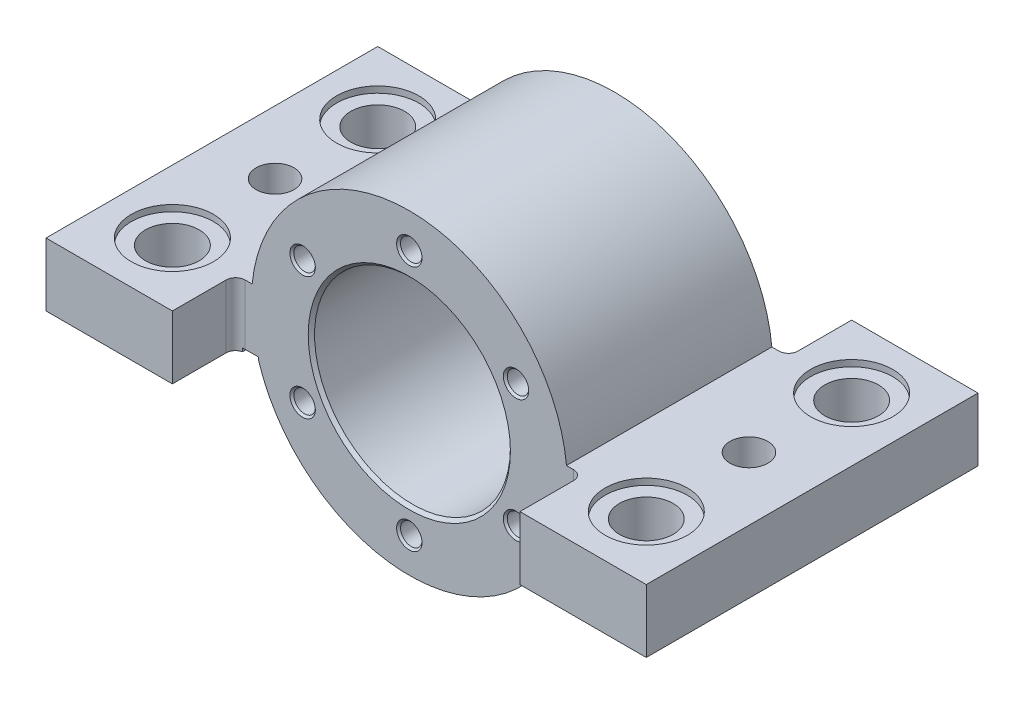
from build123d import *

# Parameters (mm, degrees)
BOSS_EXTRUDE1_DEPTH         = 52.5
BOSS_EXTRUDE1_DEPTH_BACK    = 52.5
SKETCH3_W                   = 5
SKETCH3_H                   = 10
CUT_EXTRUDE1_DEPTH          = 105
CUT_EXTRUDE2_DEPTH          = 105
CUT_EXTRUDE2_DEPTH_BACK     = 105
SKETCH5_R                   = 8.5
SKETCH5_R_2                 = 6
CUT_EXTRUDE3_DEPTH          = 105
SKETCH6_R                   = 13
CUT_EXTRUDE4_DEPTH          = 2
SKETCH7_R                   = 31
CUT_EXTRUDE5_DEPTH          = 50
SKETCH8_R                   = 28
CUT_EXTRUDE6_DEPTH          = 59
SKETCH9_R                   = 21.5
CUT_EXTRUDE7_DEPTH          = 65
CHAMFER1_SIZE               = 1
M8_TAPPED_HOLE3_D           = 6.8
M8_TAPPED_HOLE3_DEPTH       = 20
M8_TAPPED_HOLE3_CSINK_D     = 8.05
M8_TAPPED_HOLE3_CSINK_ANGLE = 90
M8_TAPPED_HOLE3_TIP         = 2.042926105
M6_TAPPED_HOLE1_D           = 5
M6_TAPPED_HOLE1_DEPTH       = 15
M6_TAPPED_HOLE1_CSINK_D     = 6.05
M6_TAPPED_HOLE1_CSINK_ANGLE = 90
M6_TAPPED_HOLE1_TIP         = 1.502151548


with BuildPart() as part:
    # Sketch1 → Boss-Extrude1 (new, two sides: drawn at the far end of the back side and taken through both)
    with BuildSketch(Plane.XY.offset(-BOSS_EXTRUDE1_DEPTH_BACK)):
        with BuildLine():
            Line((-95, -15), (-47.696960071, -15))
            ThreePointArc((-47.696960071, -15), (0, -50), (47.696960071, -15))
            Line((47.696960071, -15), (95, -15))
            Line((95, -15), (95, 5))
            Line((95, 5), (49.749371855, 5))
            ThreePointArc((49.749371855, 5), (0, 50), (-49.749371855, 5))
            Line((-49.749371855, 5), (-95, 5))
            Line((-95, 5), (-95, -15))
        make_face()
    extrude(amount=BOSS_EXTRUDE1_DEPTH + BOSS_EXTRUDE1_DEPTH_BACK)

    # Sketch3 → Cut-Extrude1 (cut)
    with BuildSketch(Plane.XY.offset(52.5)):
        with Locations((50.196960071, -19)):
            Rectangle(SKETCH3_W, SKETCH3_H)
        with Locations((-50.196960071, -19)):
            Rectangle(SKETCH3_W, SKETCH3_H)
    extrude(amount=-CUT_EXTRUDE1_DEPTH, mode=Mode.SUBTRACT)

    # Sketch4 → Cut-Extrude2 (cut, two sides: drawn at the far end of the back side and taken through both)
    with BuildSketch(Plane(origin=(0, 5, 0), x_dir=(1, 0, 0), z_dir=(0, 1, 0)).offset(-CUT_EXTRUDE2_DEPTH_BACK)):
        with BuildLine():
            Line((-52, -32.5), (52, -32.5))
            ThreePointArc((52, -32.5), (54.121320344, -33.378679656), (55, -35.5))
            Line((55, -35.5), (55, -52.5))
            Line((55, -52.5), (-55, -52.5))
            Line((-55, -52.5), (-55, -35.5))
            ThreePointArc((-55, -35.5), (-54.121320344, -33.378679656), (-52, -32.5))
        make_face()
        with BuildLine():
            Line((-55, 52.5), (55, 52.5))
            Line((55, 52.5), (55, 35.5))
            ThreePointArc((55, 35.5), (54.121320344, 33.378679656), (52, 32.5))
            Line((52, 32.5), (-52, 32.5))
            ThreePointArc((-52, 32.5), (-54.121320344, 33.378679656), (-55, 35.5))
            Line((-55, 35.5), (-55, 52.5))
        make_face()
    extrude(amount=CUT_EXTRUDE2_DEPTH + CUT_EXTRUDE2_DEPTH_BACK, mode=Mode.SUBTRACT)

    # Sketch5 → Cut-Extrude3 (cut)
    with BuildSketch(Plane(origin=(0, 5, 0), x_dir=(1, 0, 0), z_dir=(0, 1, 0))):
        with Locations(Location((-75, 32.5, 0), (0, 0, 270))):
            Circle(SKETCH5_R)
        with Locations(Location((-75, -32.5, 0), (0, 0, 90))):
            Circle(SKETCH5_R)
        with Locations(Location((75, -32.5, 0), (0, 0, 270))):
            Circle(SKETCH5_R)
        with Locations(Location((75, 32.5, 0), (0, 0, 90))):
            Circle(SKETCH5_R)
        with Locations(Location((-75, 0, 0), (0, 0, 270))):
            Circle(SKETCH5_R_2)
        with Locations(Location((75, 0, 0), (0, 0, 90))):
            Circle(SKETCH5_R_2)
    extrude(amount=-CUT_EXTRUDE3_DEPTH, mode=Mode.SUBTRACT)

    # Sketch6 → Cut-Extrude4 (cut)
    with BuildSketch(Plane(origin=(0, 5, 0), x_dir=(1, 0, 0), z_dir=(0, 1, 0))):
        with Locations(Location((-75, 32.5, 0), (0, 0, 270))):
            Circle(SKETCH6_R)
        with Locations(Location((75, 32.5, 0), (0, 0, 90))):
            Circle(SKETCH6_R)
        with Locations(Location((75, -32.5, 0), (0, 0, 270))):
            Circle(SKETCH6_R)
        with Locations(Location((-75, -32.5, 0), (0, 0, 90))):
            Circle(SKETCH6_R)
    extrude(amount=-CUT_EXTRUDE4_DEPTH, mode=Mode.SUBTRACT)

    # Sketch7 → Cut-Extrude5 (cut)
    with BuildSketch(Plane.XY.offset(32.5)):
        Circle(SKETCH7_R)
    extrude(amount=-CUT_EXTRUDE5_DEPTH, mode=Mode.SUBTRACT)

    # Sketch8 → Cut-Extrude6 (cut)
    with BuildSketch(Plane.XY.offset(32.5)):
        Circle(SKETCH8_R)
    extrude(amount=-CUT_EXTRUDE6_DEPTH, mode=Mode.SUBTRACT)

    # Sketch9 → Cut-Extrude7 (cut)
    with BuildSketch(Plane.XY.offset(32.5)):
        Circle(SKETCH9_R)
    extrude(amount=-CUT_EXTRUDE7_DEPTH, mode=Mode.SUBTRACT)

    # Chamfer1
    chamfer1_edges = [part.edges().sort_by_distance(p)[0] for p in [
        (-31, 0, 32.5),
    ]]
    chamfer(chamfer1_edges, length=CHAMFER1_SIZE)

    # M8 Tapped Hole3
    with Locations(Plane.XY.offset(32.5)):
        with Locations((-33.774990748, 19.5), (0, 39), (33.774990748, 19.5), (33.774990748, -19.5), (0, -39), (-33.774990748, -19.5), (0, 0)):
            CounterSinkHole(M8_TAPPED_HOLE3_D / 2, M8_TAPPED_HOLE3_CSINK_D / 2, depth=M8_TAPPED_HOLE3_DEPTH, counter_sink_angle=M8_TAPPED_HOLE3_CSINK_ANGLE)
            with Locations((0, 0, -(M8_TAPPED_HOLE3_DEPTH + M8_TAPPED_HOLE3_TIP / 2))):  # 118° drill point
                Cone(0, M8_TAPPED_HOLE3_D / 2, M8_TAPPED_HOLE3_TIP, mode=Mode.SUBTRACT)

    # M6 Tapped Hole1
    with Locations(Plane(origin=(0, 0, -32.5), x_dir=(-1, 0, 0), z_dir=(0, 0, -1))):
        with Locations((0, 0), (0, 39), (33.774990748, 19.5), (33.774990748, -19.5), (0, -39), (-33.774990748, -19.5), (-33.774990748, 19.5)):
            CounterSinkHole(M6_TAPPED_HOLE1_D / 2, M6_TAPPED_HOLE1_CSINK_D / 2, depth=M6_TAPPED_HOLE1_DEPTH, counter_sink_angle=M6_TAPPED_HOLE1_CSINK_ANGLE)
            with Locations((0, 0, -(M6_TAPPED_HOLE1_DEPTH + M6_TAPPED_HOLE1_TIP / 2))):  # 118° drill point
                Cone(0, M6_TAPPED_HOLE1_D / 2, M6_TAPPED_HOLE1_TIP, mode=Mode.SUBTRACT)


solid = part.part
